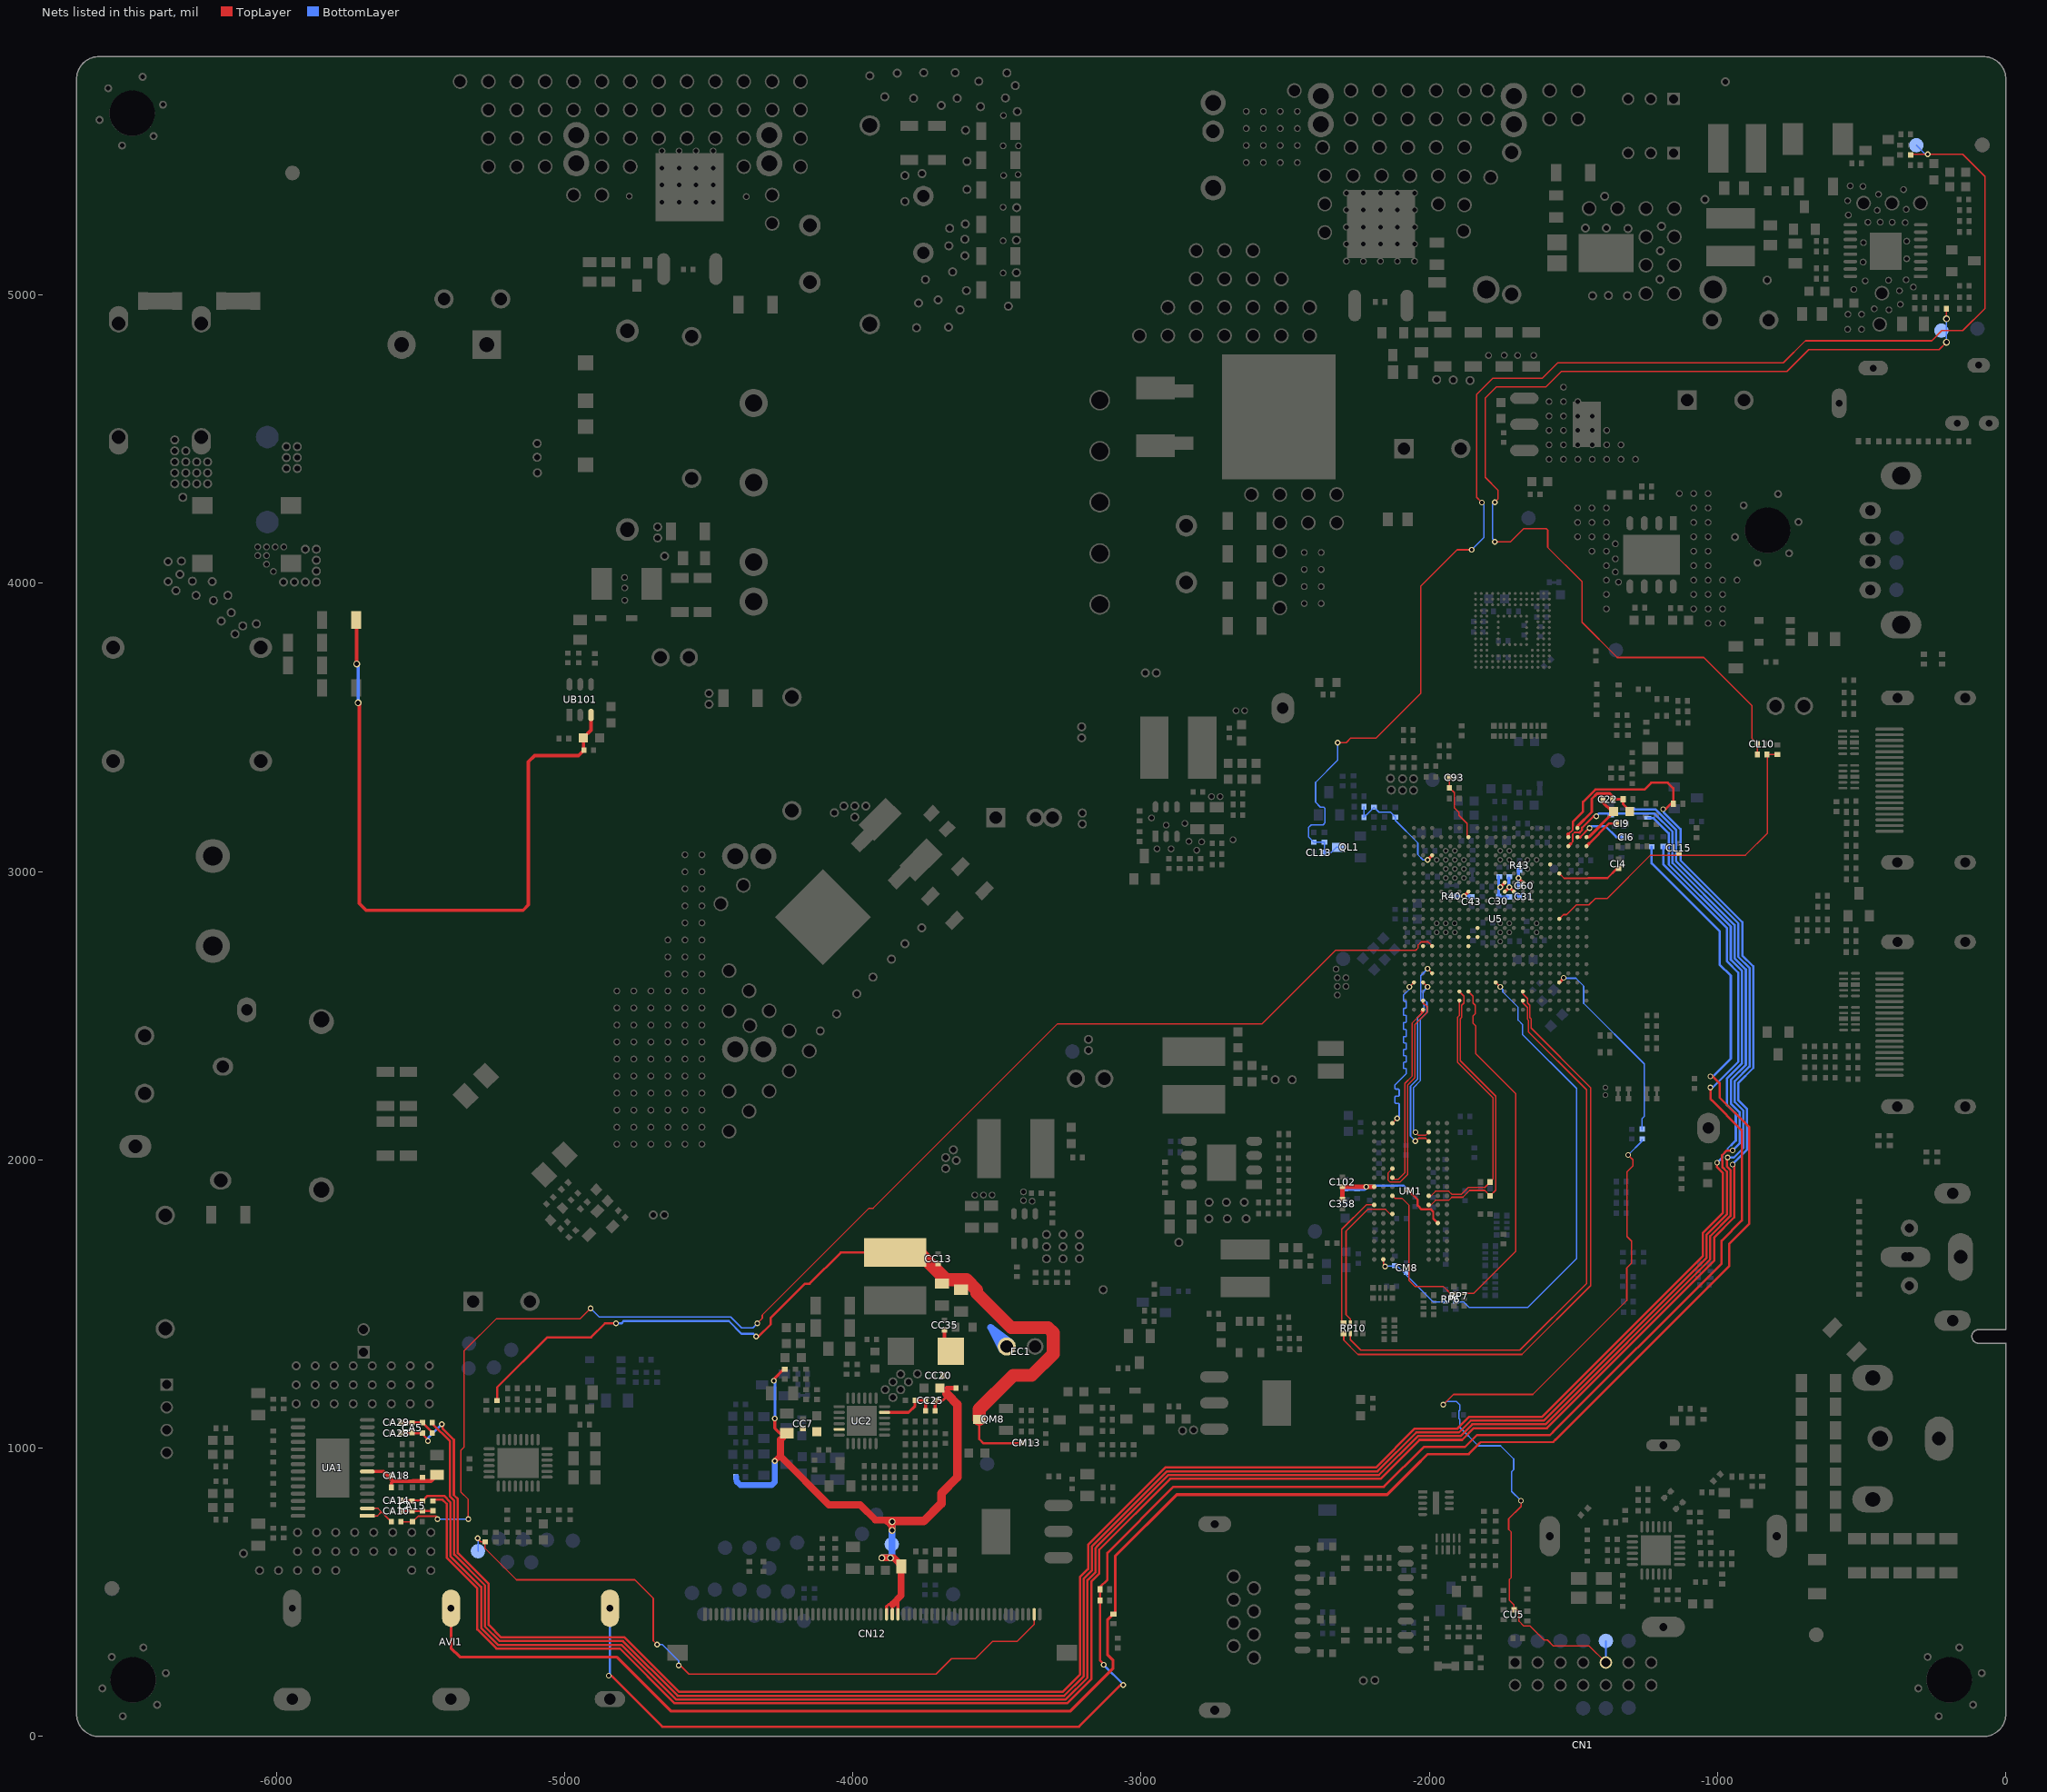
[diagram p0: the nets of this part, all layers, seen from the top]
# Altium PCB MISC84395.PcbDoc (part 11 of 26)
Units mil, origin at the board's own origin, x right, y up, seen from the top; angles counter-clockwise.
Board outline 6692.91 x 5826.77 mil, 2 copper layers (TopLayer, BottomLayer), stack 61.855 mil thick; 951 components, 565 nets, 4374 pads, 1804 vias.
Unrouted connection lines stored in the file: 1.

## Via types
v1: diameter 19.68, hole 11.81, TopLayer to BottomLayer, tented both sides, 1262 vias
v2: diameter 23.62, hole 15.75, TopLayer to BottomLayer, tented both sides, 524 vias
v3: diameter 31.5, hole 19.68, TopLayer to BottomLayer, tented both sides, 11 vias
v4: diameter 24, hole 16, TopLayer to BottomLayer, tented both sides, 6 vias
v5: diameter 19, hole 11.81, TopLayer to BottomLayer, tented both sides, 1 vias

## Nets (pads, with @x,y where several pads share a name; then routed paths per layer and width w, separated by ;. In a path a pad name is that pad's centre, name@x,y a point inside that pad or via, vN(x,y) a via of type N, cw(c..) or ccw(c..) an arc to the next point about the centre after c; other vN are vias at no path point) (continued)
A_DDR3_DQ15_IC: U5.D20 UM1.A3 | length 638.2
  TopLayer w4.92: UM1.A3@-2128.24,2127.42 v1(-2112,2143.66) ; v1(-2069.18,2599.86) U5.D20@-2053.43,2615.61
  BottomLayer w4.92: v1(-2112,2143.66) -2105.66,2150 ccw(c-2108.19,2152.52) -2104.62,2152.52 -2104.62,2192.75 ccw(c-2108.19,2192.75) -2108.18,2196.32 -2115.81,2196.32 cw(c-2115.81,2199.89) -2119.38,2199.88 -2119.38,2217.35 cw(c-2115.81,2217.35) -2115.81,2220.92 -2108.18,2220.92 ccw(c-2108.19,2224.49) -2104.62,2224.49 -2104.62,2241.96 ccw(c-2108.19,2241.96) -2108.18,2245.53 -2115.81,2245.53 cw(c-2115.81,2249.1) -2119.38,2249.1 -2119.38,2258.81 cw(c-2115.8,2258.81) -2118.33,2261.34 -2081.05,2298.62 ccw(c-2083.58,2301.14) -2080.01,2301.14 -2080.01,2313.32 ccw(c-2083.58,2313.32) -2083.58,2316.89 -2086.28,2316.89 cw(c-2086.28,2320.46) -2089.85,2320.45 -2089.85,2335.46 cw(c-2086.28,2335.46) -2086.28,2339.03 -2083.58,2339.03 ccw(c-2083.58,2342.6) -2080.01,2342.6 -2080.01,2357.61 ccw(c-2083.58,2357.61) -2083.58,2361.18 -2086.28,2361.18 cw(c-2086.28,2364.75) -2089.85,2364.75 -2089.85,2379.76 cw(c-2086.28,2379.75) -2086.28,2383.32 -2083.58,2383.32 ccw(c-2083.58,2386.89) -2080.01,2386.89 -2080.01,2401.9 ccw(c-2083.58,2401.9) -2083.58,2405.47 -2086.28,2405.47 cw(c-2086.28,2409.04) -2089.85,2409.04 -2089.85,2424.05 cw(c-2086.28,2424.05) -2086.28,2427.62 -2083.58,2427.62 ccw(c-2083.58,2431.19) -2080.01,2431.18 -2080.01,2448.65 ccw(c-2083.58,2448.65) -2083.58,2452.22 -2086.28,2452.22 cw(c-2086.28,2455.79) -2089.85,2455.79 -2089.85,2473.26 cw(c-2086.28,2473.26) -2086.28,2476.83 -2083.58,2476.83 ccw(c-2083.58,2480.4) -2080.01,2480.4 -2080.01,2497.87 ccw(c-2083.58,2497.86) -2083.58,2501.43 -2086.28,2501.43 cw(c-2086.28,2505) -2089.85,2505 -2089.85,2522.47 cw(c-2086.28,2522.47) -2086.28,2526.04 -2083.58,2526.04 ccw(c-2083.58,2529.61) -2080.01,2529.61 -2080.01,2547.08 ccw(c-2083.58,2547.08) -2083.58,2550.65 -2086.28,2550.65 cw(c-2086.28,2554.22) -2089.85,2554.21 -2089.85,2569.84 cw(c-2086.27,2569.84) -2088.81,2572.36 -2070.23,2590.94 ccw(c-2072.74,2593.47) -2069.18,2593.46 v1(-2069.18,2599.86)
A_DDR3_DQS0_IC: U5.B19 UM1.F3 | length 765.3
  TopLayer w3.94: U5.B19@-2021.94,2552.62 -2021.94,2544.74 -2008.16,2530.96 -2008.16,2511.77 -2008.65,2511.28
  TopLayer w4.92: UM1.F3@-2128.24,1969.94 -2143.99,1954.19 -2143.99,1930.57 -2136.11,1922.69 -2102.65,1922.69 -2075.09,1950.25 -2075.09,2260.29 -2050.48,2284.9 -2050.48,2469.45 -2008.65,2511.28
A_DDR3_DQS0B_IC: U5.A19 UM1.G3 | length 645.9
  TopLayer w4.92: UM1.G3@-2128.24,1938.45 -2122.33,1932.54 -2107.57,1932.54 -2084.93,1955.17 -2084.93,2241.13 -2084.93,2265.21 -2060.32,2289.82 -2060.32,2474.37 -2021.94,2512.75
  TopLayer w12: U5.A19@-2024.08,2514.89 -2021.94,2517.03 U5.A19@-2021.94,2521.12
A_DDR3_DQS1_IC: U5.E18 UM1.C7 | length 715
  TopLayer w4.92: v1@-2048.02,2065.41 -2038.18,2075.25 -2013.08,2075.25 UM1.C7@-2002.25,2064.43 ; v1(-2006.19,2662.85) U5.E18@-1990.44,2647.11
  BottomLayer w3.94: -2029.32,2552.62 -2029.81,2553.11 -2029.81,2639.23 v1(-2006.19,2662.85)
  BottomLayer w4.92: v1@-2048.02,2065.41 -2065.25,2082.64 -2065.25,2255.37 -2040.64,2279.98 -2040.64,2494.05 -2018.49,2516.2 -2018.49,2541.79 -2029.32,2552.62
  other v1: -2048.4,2065.27
A_DDR3_DQS1B_IC: U5.D19 UM1.B7 | length 616
  TopLayer w4.92: v1@-2048.02,2094.94 -2038.18,2085.1 -2013.08,2085.1 UM1.B7@-2002.25,2095.93 ; U5.D19@-2021.94,2615.61 v1(-2006.19,2599.86)
  BottomLayer w3.94: -2021.45,2559.51 -2021.94,2560 -2021.94,2584.11 v1(-2006.19,2599.86)
  BottomLayer w4.92: v1@-2048.02,2094.94 -2055.4,2102.32 -2055.4,2250.45 -2030.8,2275.06 -2030.8,2489.13 -2008.65,2511.28 -2008.65,2546.71 -2021.45,2559.51
  other v1: -2047.8,2095.43
A_DDR3_MCLK: MR301.2 U5.B15 UM1.J7 | length 929.1
  TopLayer w3.94: -1896.45,2500.45 -1895.95,2500.94 U5.B15@-1895.95,2552.62
  TopLayer w4.92: UM1.J7@-2002.25,1875.45 -1994.38,1875.45 -1978.63,1891.2 -1932.86,1891.2 -1922.04,1880.37 -1889.06,1880.37 -1865.44,1903.99 -1808.04,1903.99 -1779.81,1932.22 -1779.81,2216 -1902.84,2339.03 -1902.84,2494.05 -1896.45,2500.45
A_DDR3_MCLKZ: MR300.2 U5.C15 UM1.K7 | length 1020.9
  TopLayer w3.94: U5.C15@-1895.95,2584.12 -1880.21,2568.36 -1880.21,2544.74 -1888.08,2536.87 -1888.08,2494.05 -1888.57,2493.56
  TopLayer w4.92: UM1.K7@-2002.25,1843.96 -1994.38,1843.95 -1978.63,1859.7 -1932.86,1859.7 -1922.04,1870.53 -1884.14,1870.53 -1860.52,1894.15 -1808.04,1894.15 MR300.2@-1789.34,1875.45 -1769.97,1894.82 -1769.97,2220.92 -1893,2343.95 -1893,2489.13 -1888.57,2493.56
A_DDR3_ODT: RP10.7 UM1.K1 | length 476.9
  TopLayer w4.92: RP10.7@-2297.03,1433.03 -2303.92,1439.92 -2303.92,1759.31 -2219.28,1843.95 UM1.K1@-2191.23,1843.96
A_DDR3_ODT_IC: RP10.8 U5.C8 | length 2108.9
  TopLayer w3.94: U5.C8@-1675.48,2584.12 -1675.48,2576.24 -1659.73,2560.49 -1659.73,2544.74 -1651.86,2536.87 -1651.86,2494.05 -1649.4,2491.59
  TopLayer w4.92: RP10.8@-2297.03,1389.73 -2297.03,1374.47 -2247.82,1325.26 -1678.92,1325.26 -1440.25,1563.93 -1440.25,2250.45 -1646.94,2457.14 -1646.94,2489.13 -1649.4,2491.59
A_DDR3_RASZ: RP7.3 UM1.J3 | length 506.6
  TopLayer w4.92: UM1.J3@-2128.24,1875.45 -2119.87,1867.08 -2095.27,1867.08 -2070.17,1841.99 -2070.17,1581.16 -2063.77,1574.76 -2050.49,1561.48 -1952.05,1561.48 -1927.45,1536.87 RP7.3@-1914.65,1536.87
A_DDR3_RASZ_IC: RP7.4 U5.C14 | length 1206.7
  TopLayer w3.94: U5.C14@-1864.46,2584.12 -1848.71,2568.36 -1848.71,2544.74 -1840.84,2536.87 -1840.84,2506.85 -1841.33,2506.36
  TopLayer w4.92: RP7.4@-1871.35,1536.87 -1846.25,1536.87 -1701.07,1682.05 -1701.07,2230.77 -1838.87,2368.56 -1838.87,2464.52 -1848.71,2474.37 -1848.71,2498.97 -1841.33,2506.36
A_DDR3_RESET: CM8.2 RM10.1 RP6.3 UM1.T2 | length 280.8
  TopLayer w4.92: UM1.T2@-2159.73,1654.98 -2159.74,1636.29 v1(-2153.83,1630.38)
  BottomLayer w4.92: v1(-2153.83,1630.38) -2153.16,1631.04 -2110.52,1631.04 -1986.82,1507.34 RP6.3@-1951.56,1507.34
A_DDR3_RESET_IC: RP6.4 U5.D11 | length 1571.6
  TopLayer w4.92: U5.D11@-1769.97,2615.61 v1(-1754.22,2599.86)
  BottomLayer w4.92: RP6.4@-1908.26,1507.34 -1880.7,1507.34 -1861.01,1487.66 -1659.24,1487.66 -1489.46,1657.44 -1489.46,2247.99 -1676.47,2435 -1676.47,2469.45 -1692.01,2485 -1692.01,2529.29 -1745.36,2582.64 -1745.36,2591 v1(-1754.22,2599.86)
A_DDR3_WEZ: RP10.5 UM1.L3 | length 524.6
  TopLayer w4.92: RP10.5@-2274.4,1433.03 -2274.4,1448.29 -2289.16,1463.05 -2289.16,1752.92 -2213.87,1828.21 -2151.86,1828.21 -2136.11,1812.46 UM1.L3@-2128.24,1812.46
A_DDR3_WEZ_IC: RP10.6 U5.B8 | length 2015.9
  TopLayer w3.94: U5.B8@-1675.48,2552.62 -1675.48,2544.74 -1659.73,2528.99 -1659.73,2487.16 -1657.27,2484.7
  TopLayer w4.92: RP10.6@-2274.4,1389.73 -2274.4,1376.93 -2274.23,1376.77 -2237.49,1340.02 -1686.3,1340.02 -1455.01,1571.32 -1455.01,2243.07 -1656.78,2444.84 -1656.78,2484.21 -1657.27,2484.7
A_MVREFDQ: C102.1 C358.2 R51.1 R52.2 UM1.H1 UM1.M8 | length 557.1
  TopLayer w7.87: v1(-2075.09,1896.12) -2040.64,1861.67 -2040.64,1841.99 -2026.86,1828.21 -1994.38,1828.21 -1986.51,1820.33 -1986.51,1796.71 UM1.M8@-1970.75,1780.97
  TopLayer w15: v1(-2218.79,1906.95) UM1.H1@-2191.23,1906.95
  TopLayer w15.75: C358.2@-2301.47,1863.96 C102.1@-2301.47,1906.96 v1(-2218.79,1906.95)
  BottomLayer w7.87: v1(-2218.79,1906.95) -2214.85,1910.88 -2089.85,1910.88 v1(-2075.09,1896.12)
  BottomLayer w15.75: R52.2@-2290.85,1899.7 R51.1@-2250.28,1899.7 -2226.03,1899.7 v1(-2218.79,1906.95)
ADIM: ADIM.1 CL13.2 QL1.C RB833.2 RL1.2 RL12.1 | length 4804.7
  TopLayer w5: v1(-2318,3447) -2288.53,3447 -2272.18,3463.34 -2184.4,3463.34 -2030.38,3617.36 -2030.38,3989.5 -1903.62,4116.26 ; -1903.36,4116 v1@-1859,4116 ; v1(-1818,4280) -1836,4298 -1836,4655 -1780,4711 -1608.14,4711 -1554.65,4764.5 -772.07,4764.5 -695.57,4841 -573,4841 -257.28,4841 -222.28,4876 -150,4876 -73,4953 -73,5411 -150,5488 v1(-271,5488) -292.54,5488 ; RB833.2@-330,5485.54 -327.54,5488 -292.54,5488 ; -295.54,5488 -292.54,5488
  BottomLayer w5: RL12.1@-2366.27,3100 RL12.1@-2364,3102.27 ; -2362.25,3171.75 -2362.25,3190 ; v1(-2318,3447) -2318,3386.07 -2394.55,3309.52 -2394.75,3309.52 -2394.75,3240.74 -2377.69,3223.68 -2366.85,3223.68 -2362.25,3219.08 -2362.25,3190 ; QL1.C@-2317.03,3084.5 -2322.5,3084.5 -2341,3066 CL13.2@-2366.27,3066 -2364,3068.27 RL12.1@-2364,3102.27 ; v1(-1853,4116) -1810.55,4158.45 -1810.55,4272.55 ; ADIM.1@-311,5519 -280,5488 v1(-271,5488) ; RL12.1@-2364,3102.27 RL1.2@-2401,3102.27 -2419,3120.27 -2419,3153 -2409.91,3162.09 -2369,3162.09 -2362.25,3168.84 -2362.25,3190
AMP_L_OUT_IC: DA2.K RA13.1 U5.W3 | length 8167.6
  TopLayer w5: -1510.27,3095.79 -1502.65,3103.41 -1502.65,3129.74 -1496.65,3135.74 -1479.06,3135.74
  TopLayer w8: RA13.1@-5459.21,1086.27 -5396.97,1024.03 -5396.97,832.17 -5383.07,818.26 -5383.07,694 ; -5383.07,664.43 -5383.07,694 ; -1479.5,3135.3 -1479.06,3135.74 -1470.42,3144.38 -1470.42,3151.62 -1430.29,3191.74 v1(-1420.65,3191.74) ; v1(-948,2032.6) -968.05,2032.6 -984.44,2016.2 -984.44,1999.31 -983.16,1998.03 -983.16,1974.2 -968.42,1959.46 -968.42,1811.23 -1038.5,1741.15 -1038.5,1660.69 -1603.35,1095.84 -1856.43,1095.84 -1897.28,1055 -2045.23,1055 -2180.23,920 -2910.19,920 -3171,659.19 -3171,575.77 -3198.95,547.81 -3198.95,209.42 -3266.88,141.5 -4607.78,141.5 -4797.28,331 -5225.23,331 -5276.16,381.93 -5276.16,524.31 -5383.07,631.22 -5383.07,694
  TopLayer w12: U5.W3@-1518,3088.05 -1510.27,3095.79
  BottomLayer w8: v1(-1420.65,3191.74) -1410.65,3201.74 -1220.1,3201.74 -1156.8,3138.44 -1156.8,3030.23 -941.34,2814.77 -941.34,2699.39 -902.3,2660.36 -902.3,2329.57 -954,2277.88 -954,2195.54 -924,2165.54 -924,2056.6 v1(-948,2032.6)
AMP_LINN: CA5.2 CA28.2 GND_JP2.JP_1K RA12.2 | length 7881.1
  TopLayer w8: CA28.2@-5567.13,1051.94 RA12.2@-5494.86,1051.94 ; RA12.2@-5492.68,1053 -5492.68,1048.73 v1@-5471.44,1027.5 ; v1@-5422.94,1083 -5422.94,1068.38 -5383.97,1029.41 -5383.97,837.55 -5370.07,823.65 -5370.07,636.61 -5263.16,529.7 -5263.16,387.31 -5219.85,344 -5053,344 -4791.9,344 -4602.4,154.5 -3272.26,154.5 -3212.3,214.47 -3212.3,552.86 -3184,581.15 -3184,664.58 -2915.58,933 -2185.62,933 -2050.62,1068 -1902.66,1068 -1861.82,1108.84 -1608.73,1108.84 -1051.5,1666.08 -1051.5,1746.54 -981.42,1816.62 -981.42,1954.08 -1002,1974.66 v1(-1002,1990)
  BottomLayer w5: -984.44,2012.8 -984.44,2014.92 -965.34,2034.02 -965.34,2039.78 -955.18,2049.94 -954.06,2049.94 -952.56,2051.44
  BottomLayer w8: -5473.94,1035 v1(-5425.94,1083) ; GND_JP2.JP_1K@-1240.4,3185 -1221.74,3185 -1169.8,3133.06 -1169.8,3024.85 -954.34,2809.38 -954.34,2694 -915.3,2654.97 -915.3,2334.96 -967,2283.26 -967,2190.15 -937,2160.15 -937,2067 -952.56,2051.44 ; v1(-1002,1990) -984.44,2007.56 -984.44,2012.8
  other v1: -5473.94,1025
AMP_LINP: CA5.1 CA29.2 RA12.1 RA13.2 | length 124.3
  TopLayer w8: CA29.2@-5567.13,1088.94 CA29.2@-5567.07,1088.94 ; CA29.2@-5567.07,1089 RA13.2@-5492.68,1089 -5459.21,1055.54 RA12.1@-5459.21,1053
AMP_MUTE: RA32.1 UA1.1 UA1.2 | length 154.9
  TopLayer w5: UA1.1@-5684.07,765.6 -5648.63,765.6 -5636.77,777.46 ; UA1.2@-5684.07,791.19 -5646.85,791.19 RA32.1@-5600.6,744.94
AMP_MUTE_IC: RA31.2 RA32.2 U5.H18 | length 4857.1
  TopLayer w5: RA32.2@-5567.13,744.94 RA31.2@-5527.33,744.94 -5507.96,764.31 -5444.26,764.31 ; v1(-5333.94,754) -5333.94,822.17 -5359.47,847.7 -5359.47,992.67 -5349,1003.14 -5349,1336.67 -5236.17,1449.5 -4945.5,1449.5 v1(-4909.5,1485.5) ; v1(-4331.09,1433.06) -4314.04,1450.1 -4314.04,1462.04 -3943.75,1832.33 -3929.61,1832.33 -3290.94,2471 -2581.11,2471 -2325.1,2727.01 -2047.39,2727.01 -2038.85,2735.55 -2038.85,2745.31 -2027.98,2756.18 -2005.03,2756.18 U5.H18@-1990.44,2741.6
  BottomLayer w5: v1(-5440.94,754) v1(-5333.94,754) ; v1(-4909.5,1485.5) -4879.5,1455.5 -4827.77,1455.5 -4423.84,1455.5 -4385.9,1417.56 -4346.58,1417.56 v1(-4331.09,1433.06)
AMP_R_OUT_IC: DA1.K RA6.1 U5.Y3 | length 8199.4
  TopLayer w6: -1518,3129.71 -1502.65,3145.06 -1502.65,3161.74
  TopLayer w8: RA6.1@-5456.6,816.67 -5451.74,821.53 -5423.11,821.53 -5409.07,807.49 -5409.07,620.45 -5302.16,513.54 -5302.16,371.16 -5236,305 -4808.05,305 -4618.55,115.5 -3256.11,115.5 -3172.95,198.66 -3172.95,537.05 -3145,565 -3145,648.42 -2899.42,894 -2169.46,894 -2034.46,1029 -1886.51,1029 -1845.66,1069.84 -1592.58,1069.84 -1012.5,1649.92 -1012.5,1730.38 -942.42,1800.46 -942.42,1979 v1@-948.42,1985 ; -1502.25,3158.05 -1502.25,3172.14 -1466.65,3207.74 -1466.65,3242.11 -1424.18,3284.58 -1401,3284.58 ; -1416.3,3284.58 -1401,3284.58 ; v1(-1189.24,3215.91) -1187.84,3217.3 -1179.52,3217.3 -1154.16,3242.67 -1154.16,3289.19 -1173.21,3308.24 -1230.76,3308.24 -1254.42,3284.58 -1401,3284.58
  TopLayer w12: U5.Y3@-1518,3119.55 -1518,3129.71
  BottomLayer w8: v1@-1187.4,3216.9 -1187.4,3205.81 -1128.8,3147.21 -1128.8,3039 -914.46,2824.66 -914.46,2709.28 -876.3,2671.12 -876.3,2318.8 -928,2267.11 -928,2206.31 -898,2176.31 -898,2035.42 v1@-948.42,1985
  other v1: -948.02,1984.2
AMP_RINN: CA14.2 CA15.1 GND_JP1.JP_1K RA5.1 | length 7856
  TopLayer w8: CA14.2@-5567.13,818.96 -5494.83,818.96 RA5.1@-5492.6,816.72 -5474.79,834.53 -5417.72,834.53 -5396.07,812.88 -5396.07,710 ; -5396.07,659.05 -5396.07,710 ; v1@-962,2012 v1(-965.6,2008.4) -967.26,2006.74 -967.26,1976.69 -955.42,1964.84 -955.42,1805.85 -1025.5,1735.77 -1025.5,1655.31 -1597.97,1082.84 -1851.05,1082.84 -1891.89,1042 -2039.85,1042 -2174.85,907 -2904.81,907 -3150.38,661.42 -3158,653.81 -3158,570.38 -3185.95,542.43 -3185.95,204.04 -3261.49,128.5 -4613.17,128.5 -4802.67,318 -5230.62,318 -5289.16,376.54 -5289.16,518.93 -5396.07,625.84 -5396.07,710
  BottomLayer w8: GND_JP1.JP_1K@-1300.4,3217.4 -1297.74,3214.74 -1214.72,3214.74 -1143.8,3143.83 -1143.8,3035.62 -928.34,2820.15 -928.34,2704.77 -889.3,2665.74 -889.3,2324.19 -941,2272.49 -941,2200.92 -911,2170.92 -911,2040.8 -943.4,2008.4 v1(-965.6,2008.4)
AMP_RINP: CA10.2 CA15.2 RA5.2 RA6.2 | length 111.1
  TopLayer w8: CA10.2@-5567.13,781.96 -5457.84,781.96 RA6.2@-5456.6,783.21
AUVGA_IC: C21.2 C22.2 U5.Y1 | length 193.3
  TopLayer w10: U5.Y1@-1455.01,3119.55 -1447.37,3119.55 C21.2@-1366.46,3200.47 ; C22.2@-1397.51,3250.74 -1397.5,3239.47 -1366.77,3208.74 C21.2@-1360.58,3208.74 -1358.58,3208.74 C21.2@-1358.58,3200.47
AUVRM_IC: C21.1 C22.1 L3.1 U5.AA2 | length 304.9
  TopLayer w10: U5.AA2@-1486.5,3151.04 -1486.5,3156.88 -1436.65,3206.74 -1436.65,3252.32 -1418.38,3270.58 -1373.62,3270.58 -1364.04,3261.01 C22.1@-1364.04,3250.74 L3.1@-1327.77,3250.74 -1327.77,3233.55 C21.1@-1302.96,3208.74
AV/YPBPR_L_IN_IC: CI6.2 U5.Y2 | length 181.5
  TopLayer w7: -1477.05,3119.55 v1@-1445.86,3150.74
  TopLayer w12: U5.Y2@-1486.5,3119.55 -1477.05,3119.55
  BottomLayer w8: v1(-1444.65,3150.74) -1438.8,3156.58 -1388.49,3156.58 -1351.65,3119.74 CI6.2@-1334.38,3119.74
AV/YPBPR_R_IN_IC: CI9.2 U5.W1 | length 159.6
  TopLayer w5: U5.W1@-1455.01,3088.05 U5.W1@-1450.96,3088.05
  TopLayer w8: -1446.59,3096.47 -1376.32,3166.74 CI9.2@-1350.24,3166.74 -1368.45,3166.74
  TopLayer w12: U5.W1@-1455.01,3088.05 -1446.59,3096.47
AV_CVBS_IN_IC: CI4.1 U5.T4 | length 223.9
  TopLayer w5: U5.T4@-1547.17,2993.56 U5.T4@-1549.5,2993.56 -1532.59,2976.65 -1443.65,2976.65
  TopLayer w8: -1447.75,2977.56 -1382.1,2977.56 CI4.1@-1351.65,3008.01
AV_L_IN: AVI1.3 DI2.K RI7.2 | length 7245
  TopLayer w7: -1833.4,1009.98 -1825.35,1018.03 -1822.04,1021.34 -1570.37,1021.34 -1569.87,1021.84
  TopLayer w8: -2030.36,955.36 -2005.71,980 -1863.38,980 -1825.35,1018.03 ; -1569.87,1021.84 -1562.63,1029.08 -960.5,1631.21 -960.5,1708.84 -890,1779.34 -890,2113.23 -993.16,2216.39 -993.16,2266 -1016.78,2289.63 v1(-1025.05,2289.63)
  TopLayer w10: AVI1.3@-5393.7,444.88 -5393.7,306.7 -5363,276 -4819.36,276 -4631.86,88.5 -3244.93,88.5 -3097.96,235.46 -3097.96,265.75 -3116.83,284.61 -3116.83,303 -3116.83,404.27 -3096.36,424.73 DI2.K@-3096,424.73 -3090,430.73 -3090,625.64 -2876.64,839 -2146.71,839 -2030.36,955.36
  BottomLayer w8: RI7.2@-1228.65,3086.01 -1228.65,3028.54 -993.34,2793.23 -993.34,2677.85 -954.3,2638.82 -954.3,2351.11 -1015.79,2289.63 v1(-1025.05,2289.63)
AV_R_IN: AVI1.5 DI4.K DI04.K RI11.2 | length 6872.4
  TopLayer w7: -2018.66,1004.5 -1876.36,1004.5 -1835.51,1045.34 -1581.73,1045.34 -1571.98,1055.09
  TopLayer w8: v1(-4846.5,211) -4837.8,211 -4661.3,34.5 -3215.49,34.5 -3070.99,179 v1(-3062,179) ; v1(-3130,249) -3130,252.27 -3142.83,265.1 -3142.83,464.91 -3142.73,465 -3142.73,517.77 -3117,543.5 -3117,636.82 -2887.82,866 -2157.86,866 -2020.18,1003.68 ; -1571.98,1055.09 -986.5,1640.57 -986.5,1719.61 -916,1790.11 -916,2102.46 -1020.9,2207.37 -1024.74,2211.2 -1024.74,2250.74 v1(-1025,2251)
  BottomLayer w8: v1(-4846.5,211) -4842.52,214.98 AVI1.5@-4842.52,444.88 ; v1(-3130,249) -3062,181 v1(-3062,179) ; RI11.2@-1188.65,3087.01 -1188.65,3025.31 -967.34,2804 -967.34,2688.62 -928.3,2649.59 -928.3,2340.34 -1017.65,2251 v1(-1025,2251)
AVCC: CA18.1 RA8.1 RA25.2 RA27.2 UA1.7 | length 288.1
  TopLayer w12: UA1.7@-5684.07,919.15 -5628.66,919.15 -5594.68,885.16 ; RA8.1@-5600.6,863.93 -5600.6,879.24 -5594.68,885.16 ; -5526.51,885.16 -5594.68,885.16
  TopLayer w15: -5526.51,886.34 -5464.1,886.34 RA27.2@-5442.6,907.85
AVDD: AVDD.1 CC4.1 CC7.2 CC19.1 CC20.2 CC22.1 CC25.2 CC35.1 CN12.33 CN12.34 CN12.35 DC1.K EC1.1 pad.VIA5@-3864,715 pad.VIA5@-3864,745 pad.VIA5@-3869,619.5 pad.VIA5@-3899,619.5 RC1.1 RC9.2 RC16.2 RC18.2 RC19.2 UC2.5 | length 2488.3
  TopLayer w10: v1(-4273.58,1233.45) -4273.58,1239.85 -4239.86,1273.57 RC9.2@-4236.24,1273.57 ; v1(-4270.46,1102.82) -4270.46,1069.46 -4252.91,1051.91 ; CN12.33@-3882.79,423.98 -3882.79,451.39 -3875.8,458.38 -3863.11,458.38 CN12.34@-3863.11,423.98 ; CN12.35@-3843.42,423.98 -3843.42,477.07 ; RC16.2@-3714.27,1130 CC25.2@-3714.27,1166 ; -3696,1166 CC25.2@-3714.27,1166 ; -3669.62,1184.62 -3688.23,1166 CC25.2@-3714.27,1166
  TopLayer w12: DC1.K@-3682,1358.01 CC35.1@-3682,1410.27
  TopLayer w15: -3674.23,1208.27 RC18.2@-3642,1208.27
  TopLayer w20: v1(-4270.31,955.31) -4254.74,970.89
  TopLayer w24: RC1.1@-4229,1051.91 -4250.82,1030.09 -4250.82,970.89 -4083.52,803.59 -3974.39,803.59 -3921.54,750.75 -3883.75,750.75 -3864,731 pad.VIA5@-3864,715 ; pad.VIA5@-3899,619.5 -3858.53,619.5 CC19.1@-3828.03,589 ; -3863.11,458.38 -3832.03,489.46 CC19.1@-3832.03,590 CC19.1@-3832.03,570.97
  TopLayer w30: -3879.04,747.75 -3753.17,747.75 -3693,807.91 -3693,843.4 -3637.4,899 -3637.4,1152.4 -3669.62,1184.62 -3674.5,1189.5 ; DC1.K@-3659.99,1311.01 DC1.K@-3659.99,1332
  BottomLayer w10: v1@-4269.65,1103.63 v1@-4269.65,1229.52
  BottomLayer w20: RC19.2@-4404,900.19 -4404,885.73 -4390.21,871.94 -4280.86,871.94 -4270.31,882.49 v1(-4270.31,955.31)
  BottomLayer w24: pad.VIA5@-3899,619.5 pad.VIA5@-3869,619.5 -3864,624.5 -3864,697 ; pad.VIA5@-3864,713 -3864,697 ; pad.VIA5@-3864,745 pad.VIA5@-3864,715 -3864,697
AVDD_AU33: C31.2 R39.2 U5.P9 U5.P10 | length 122.8
  TopLayer w10: U5.P10@-1738.47,2930.57 v1(-1722.72,2946.32) U5.P9@-1706.98,2930.57
  BottomLayer w10: R39.2@-1723.97,2978.12 -1723.97,2947.56 v1(-1722.72,2946.32) -1705.32,2928.91 ; -1705.28,2928.91 -1690.97,2914.6 C31.2@-1690.97,2913.58
AVDD_DDR_VBN_A: U5.H14
AVDD_DDR_VBN_B: U5.J14
AVDD_DDR_VBP_A: U5.J13
AVDD_DDR_VBP_B: U5.K13
AVDD_DMPLL: C30.2 D5.K R38.2 U5.R10 | length 125.3
  TopLayer w10: v1(-1754.22,2946.32) U5.R10@-1738.47,2962.07
  BottomLayer w10: R38.2@-1759.97,2982.62 -1759.71,2982.36 -1759.71,2914.08 -1757.71,2912.08 D5.K@-1726.21,2912.08
AVDD_FB: CC25.1 RC16.1 RC17.2 UC2.17 | length 206.8
  TopLayer w10: UC2.17@-3890,1124.45 -3806.55,1124.45 -3784.27,1146.73 RC17.2@-3784.27,1166 -3747.73,1166 RC16.1@-3747.73,1130
AVDD_PLL: C60.2 R43.2 R43.3 U5.R8 | length 73.1
  TopLayer w10: v1(-1691.23,2977.82) U5.R8@-1675.48,2962.07
  BottomLayer w10: C60.2@-1691.23,2954.19 v1(-1691.23,2977.82) R43.2@-1691.23,3005.06
AVDD_SOURCE: CC8.1 CC12.1 CC13.2 CM13.1 LC1.1 QM8.D RW3.1 | length 2928.4
  TopLayer w8: RW3.1@-5234,1165.73 -5234,1210.9 -5059.9,1385 -4908,1385 -4860,1433 v1(-4821.5,1433) ; v1(-4335.47,1387.57) -4327.21,1387.57 -4284.75,1430.03 -4284.75,1452.45 -4166.57,1570.63 -4150.04,1570.63 -4041.8,1678.87 LC1.1@-3853,1678.87 ; QM8.D@-3561.28,1100 -3561.28,1031.28 -3547,1017 CM13.1@-3414.73,1017
  TopLayer w45: LC1.1@-3766.38,1678.87 -3766.38,1674.28 -3676.35,1584.25 -3605.82,1584.25 -3569.89,1548.32 -3569.89,1537.74 -3450.15,1418 -3322.74,1418 -3305,1400.26 -3305,1326.92 -3379.26,1252.66 -3443.68,1252.66 -3561.28,1135.06 QM8.D@-3561.28,1100
  BottomLayer w8: v1(-4821.5,1433) -4803,1433 -4795,1441 -4429.85,1441 -4385.85,1397 -4344.9,1397 v1(-4335.47,1387.57)
AVDDL_MOD: C43.2 R40.2 R40.3 U5.P14 | length 67.9
  TopLayer w10: v1(-1880.2,2914.82) U5.P14@-1864.46,2930.57
  BottomLayer w10: R40.2@-1905.98,2914.51 v1@-1880.2,2914.51 ; v1(-1880.2,2914.82) C43.2@-1860.33,2914.82
BL_DIM_OUT_IC: RL4.1 RL5.2 RL9.2 RL11.1 U5.V18 | length 401.9
  TopLayer w10: v1(-2006.19,3040.81) U5.V18@-1990.44,3056.56
  BottomLayer w5: RL9.2@-2229,3189.27 -2225.46,3189.27 RL4.1@-2192,3222.73 -2174.89,3205.63 -2134.63,3205.63 RL11.1@-2118,3189 -2118,3177.37 -2040,3099.37 -2040,3058.81 -2022,3040.81 v1(-2006.19,3040.81) ; RL9.2@-2227.27,3188 RL5.2@-2227.27,3225
BL_ON: BL_ON.1 CL10.2 RB802.1 RL6.1 | length 3772.1
  TopLayer w5: v1(-1773,4144) -1718.55,4144 -1673.05,4189.5 -1594.5,4189.5 -1589.33,4184.33 -1589.33,4124.1 -1470.65,4005.41 -1470.65,3864.65 -1348.52,3742.52 -1048.31,3742.52 -880.46,3574.68 -880.46,3460.88 CL10.2@-862.57,3443 RL6.1@-862.57,3406 ; v1(-1773,4281) -1761.66,4292.34 -1761.66,4322.66 -1806,4367 -1806,4642.57 -1767.57,4681 -1595.72,4681 -1542.22,4734.5 -759.65,4734.5 -684.14,4810 -232,4810 v2(-206,4836) ; v2@-206.27,4917.27 RB802.1@-206.27,4952.32
  BottomLayer w5: v1(-1773,4281) -1780.55,4273.45 -1780.55,4154.93 v1@-1771.91,4146.28 ; v2@-206,4846 v2(-206,4917)
BL_ON_IC: CL15.2 RL6.2 RL8.2 U5.L4 | length 1153.9
  TopLayer w5: U5.L4@-1549.5,2836.08 -1534.91,2850.67 -1524.04,2850.67 -1490.22,2884.49 -1446.45,2884.49 -1424.17,2906.77 -1383.07,2906.77 -1232.97,3056.87 -903.9,3056.87 -826.93,3133.85 RL6.2@-826.93,3408 ; RL6.2@-826.66,3406.27 RL8.2@-792.83,3406.27
BRO: CB111.2 RB104.2 RB142.1 UB101.3 | length 2431.2
  TopLayer w11.81: RB142.1@-5722.89,3873 -5721,3871.11 v2(-5721,3720) ; v2(-5716,3585) -5711.49,3580.49 -5711.49,2889.32 -5687.98,2865.81 -5143.96,2865.81 -5125.22,2884.56 -5125.22,3380.79 -5103.7,3402.3 -4951.49,3402.3 RB104.2@-4932.49,3421.3 -4934.3,3423.11 CB111.2@-4934.3,3464.3 -4908.09,3490.51 UB101.3@-4908.09,3543
  BottomLayer w11.81: v2(-5721,3720) -5716,3715 v2(-5716,3585)
BT_HOST_WAKE_IC: U5.U5
BT_RESET: BT_RST.1 CN1.9 CU5.2 R1.1 | length 2833.2
  TopLayer w5: v1(-1952,1151) -1916.36,1186.64 -1641.12,1186.64 -1315.17,1512.59 -1315.17,1625.48 -1298.66,1642 -1298.66,1718.32 -1314.67,1734.33 -1314.67,1958.47 -1294.17,1978.97 -1294.17,2000.64 v1(-1310.32,2016.79) ; CU5.2@-1707.84,438.12 -1706.34,436.62 -1693.41,436.62 -1689,432.22 -1689,399.98 -1672.79,383.77 -1650.77,383.77 -1601.72,334.72 -1590.4,334.72 -1569.58,313.89 -1444.95,313.89 CN1.9@-1387.79,256.74 ; CU5.2@-1706.34,439.62 -1706.34,456.55 -1722.67,472.88 -1722.67,544.82 -1715.67,551.82 -1715.67,709.33 -1724.79,718.45 -1724.79,755.69 -1682,798.47 v1(-1682,818)
  BottomLayer w5: v1(-1952,1151) -1941,1162 -1906.47,1162 -1894.66,1150.18 -1894.66,1131.92 -1897.63,1128.95 -1897.63,1103.05 -1894.66,1100.08 -1894.66,1072.42 -1830.74,1008.5 -1753.27,1008.5 -1707.66,962.89 -1707.66,925.63 -1714.34,918.95 -1714.34,850.34 v1(-1682,818) ; CN1.9@-1387.79,256.74 BT_RST.1@-1387.8,331.95 ; v1(-1310.32,2016.79) -1262,2065.1 R1.1@-1262,2071.27
BT_RESET_IC: R1.2 U5.D4 | length 691.7
  TopLayer w5: U5.D4@-1549.5,2615.61 U5.D4@-1549.22,2615.61
  TopLayer w10: U5.D4@-1549.5,2615.61 -1533.99,2631.12 v1(-1533.99,2631.6)
  BottomLayer w5: v1@-1533.99,2630.01 -1491.83,2630.01 -1464.91,2603.09 -1464.91,2543.29 -1254.3,2332.68 -1254.3,2150.76 -1262,2143.06 R1.2@-1262,2104.73
BT_UART_NEN_IC: U5.H19
C-MCKE: C93.2 R47.2 U5.Y14 | length 234.1
  TopLayer w5: C93.2@-1930.02,3326.48 R47.2@-1930.01,3290.48 -1913.64,3274.11 -1913.64,3220.78 -1897.82,3204.96 -1897.82,3195.06 -1869.04,3166.28 -1869.04,3124.14 U5.Y14@-1864.46,3119.55
CLK1: CLK1.1 CN12.59 RG91.2 | length 2399
  TopLayer w5: v1(-5301.2,688.17) -5301.2,685.94 -5290.03,674.77 RG91.2@-5275.51,674.77 ; -5275.51,656.1 RG91.2@-5275.51,674.77 ; v1(-4679,319) -4692.34,332.34 -4692.34,479.48 -4756.36,543.5 -5166.92,543.5 -5275.51,652.1 RG91.2@-5275.51,674.77 ; v1(-4604,246.5) -4598.53,246.5 -4568.5,216.47 -3711.28,216.47 -3657.51,270.24 -3574.73,270.24 -3514.73,330.24 -3430.11,330.24 -3370.98,389.37 CN12.59@-3370.98,418.08
  BottomLayer w5: CLK1.1@-5300.26,643 v1@-5300.26,687.23 ; v1(-4679,319) -4660.47,319 -4604,262.53 v1(-4604,246.5)